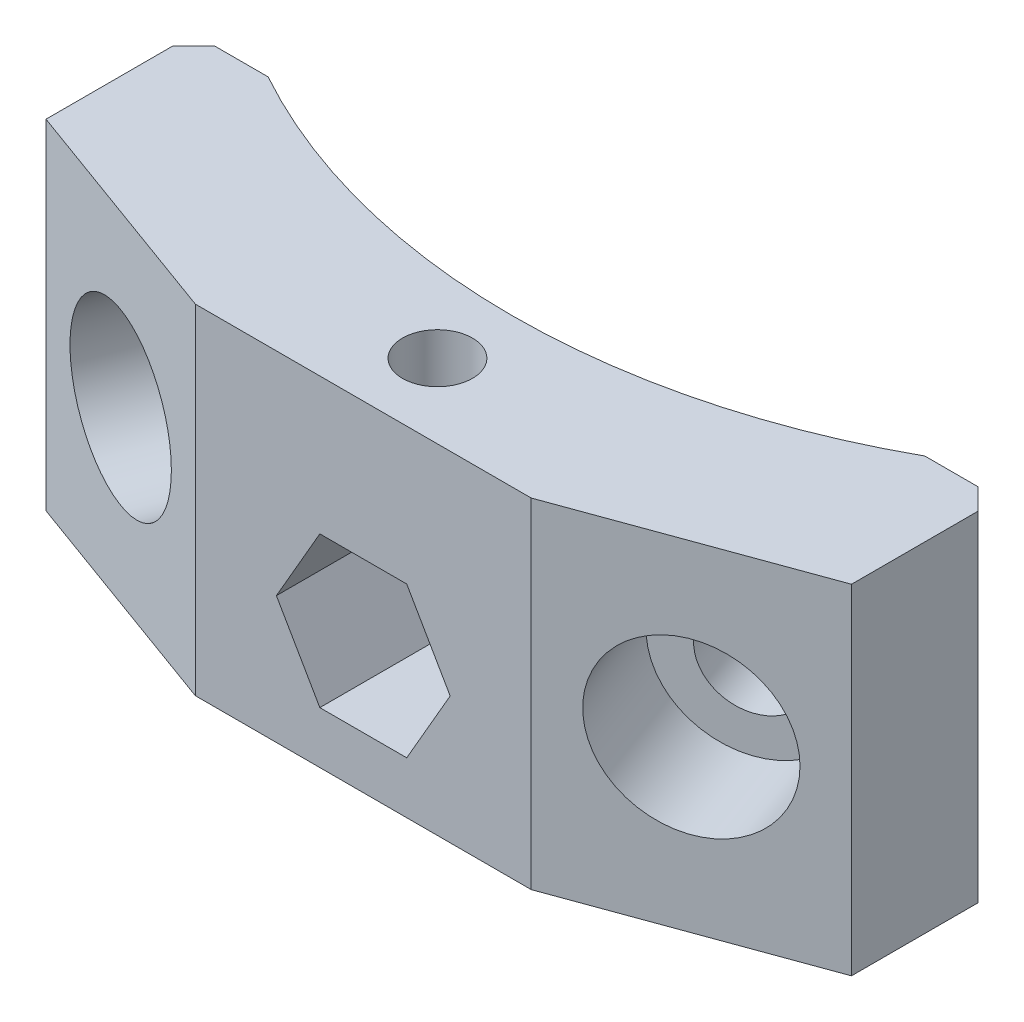
from build123d import *

# Parameters (mm, degrees)
BOSS_EXTRUDE1_DEPTH                                  = 8
CUT_EXTRUDE2_DEPTH                                   = 24.366642891
M4_TAPPED_HOLE1_D                                    = 3.3
M4_TAPPED_HOLE1_DEPTH                                = 11.5
M4_TAPPED_HOLE1_TIP                                  = 0.991420021
HOLE_SIZE_PER_SOCKET_HEAD_CAP_SCREW_TYPE_D           = 4.5
HOLE_SIZE_PER_SOCKET_HEAD_CAP_SCREW_TYPE_CBORE_D     = 8
HOLE_SIZE_PER_SOCKET_HEAD_CAP_SCREW_TYPE_CBORE_DEPTH = 5
CHAMFER2_SIZE                                        = 1


with BuildPart() as part:
    # Sketch1 → Boss-Extrude1 (new, symmetric)
    with BuildSketch(Plane(origin=(0, 0, 0), x_dir=(1, 0, 0), z_dir=(0, 1, 0))):
        with BuildLine():
            Line((-7.922147119, -39), (7.922147119, -39))
            Line((7.922147119, -39), (19, -34.967991292))
            Line((19, -34.967991292), (19, -28))
            Line((19, -28), (15.491933385, -28))
            ThreePointArc((15.491933385, -28), (0, -32), (-15.491933385, -28))
            Line((-15.491933385, -28), (-19, -28))
            Line((-19, -28), (-19, -34.967991292))
            Line((-19, -34.967991292), (-7.922147119, -39))
        make_face()
    extrude(amount=BOSS_EXTRUDE1_DEPTH, both=True)

    # Sketch2 → Cut-Extrude2 (cut, through all)
    with BuildSketch(Plane.XY.offset(39)):
        Polygon((4.099186911, -2), (2.049593456, 1.55), (-2.049593456, 1.55), (-4.099186911, -2), (-2.049593456, -5.55), (2.049593456, -5.55), align=None)
    extrude(amount=-CUT_EXTRUDE2_DEPTH, mode=Mode.SUBTRACT)

    # M4 Tapped Hole1
    with Locations(Plane(origin=(0, 8, 0), x_dir=(1, 0, 0), z_dir=(0, 1, 0))):
        with Locations((0, -35.5)):
            Hole(M4_TAPPED_HOLE1_D / 2, depth=M4_TAPPED_HOLE1_DEPTH)
            with Locations((0, 0, -(M4_TAPPED_HOLE1_DEPTH + M4_TAPPED_HOLE1_TIP / 2))):  # 118° drill point
                Cone(0, M4_TAPPED_HOLE1_D / 2, M4_TAPPED_HOLE1_TIP, mode=Mode.SUBTRACT)

    # Hole size per socket head cap screw type 2 (through all)
    with Locations(Plane(origin=(-13.461073559, 0, 36.983995646), x_dir=(0.9396926207859081, 0, 0.34202014332566943), z_dir=(-0.34202014332566943, 0, 0.9396926207859081))):
        with Locations((0, 0)):
            hole_size_per_socket_head_cap_screw_type = CounterBoreHole(HOLE_SIZE_PER_SOCKET_HEAD_CAP_SCREW_TYPE_D / 2, HOLE_SIZE_PER_SOCKET_HEAD_CAP_SCREW_TYPE_CBORE_D / 2, HOLE_SIZE_PER_SOCKET_HEAD_CAP_SCREW_TYPE_CBORE_DEPTH)

    # Mirror3: Hole size per socket head cap screw type 2 across plane
    add(hole_size_per_socket_head_cap_screw_type.mirror(Plane(origin=(0, 0, 0), x_dir=(0, 0, 1), z_dir=(1, 0, 0))), mode=Mode.SUBTRACT)

    # Chamfer2
    chamfer2_edges = [part.edges().sort_by_distance(p)[0] for p in [
        (-19, 0, 28),
        (19, 0, 28),
    ]]
    chamfer(chamfer2_edges, length=CHAMFER2_SIZE)


solid = part.part
